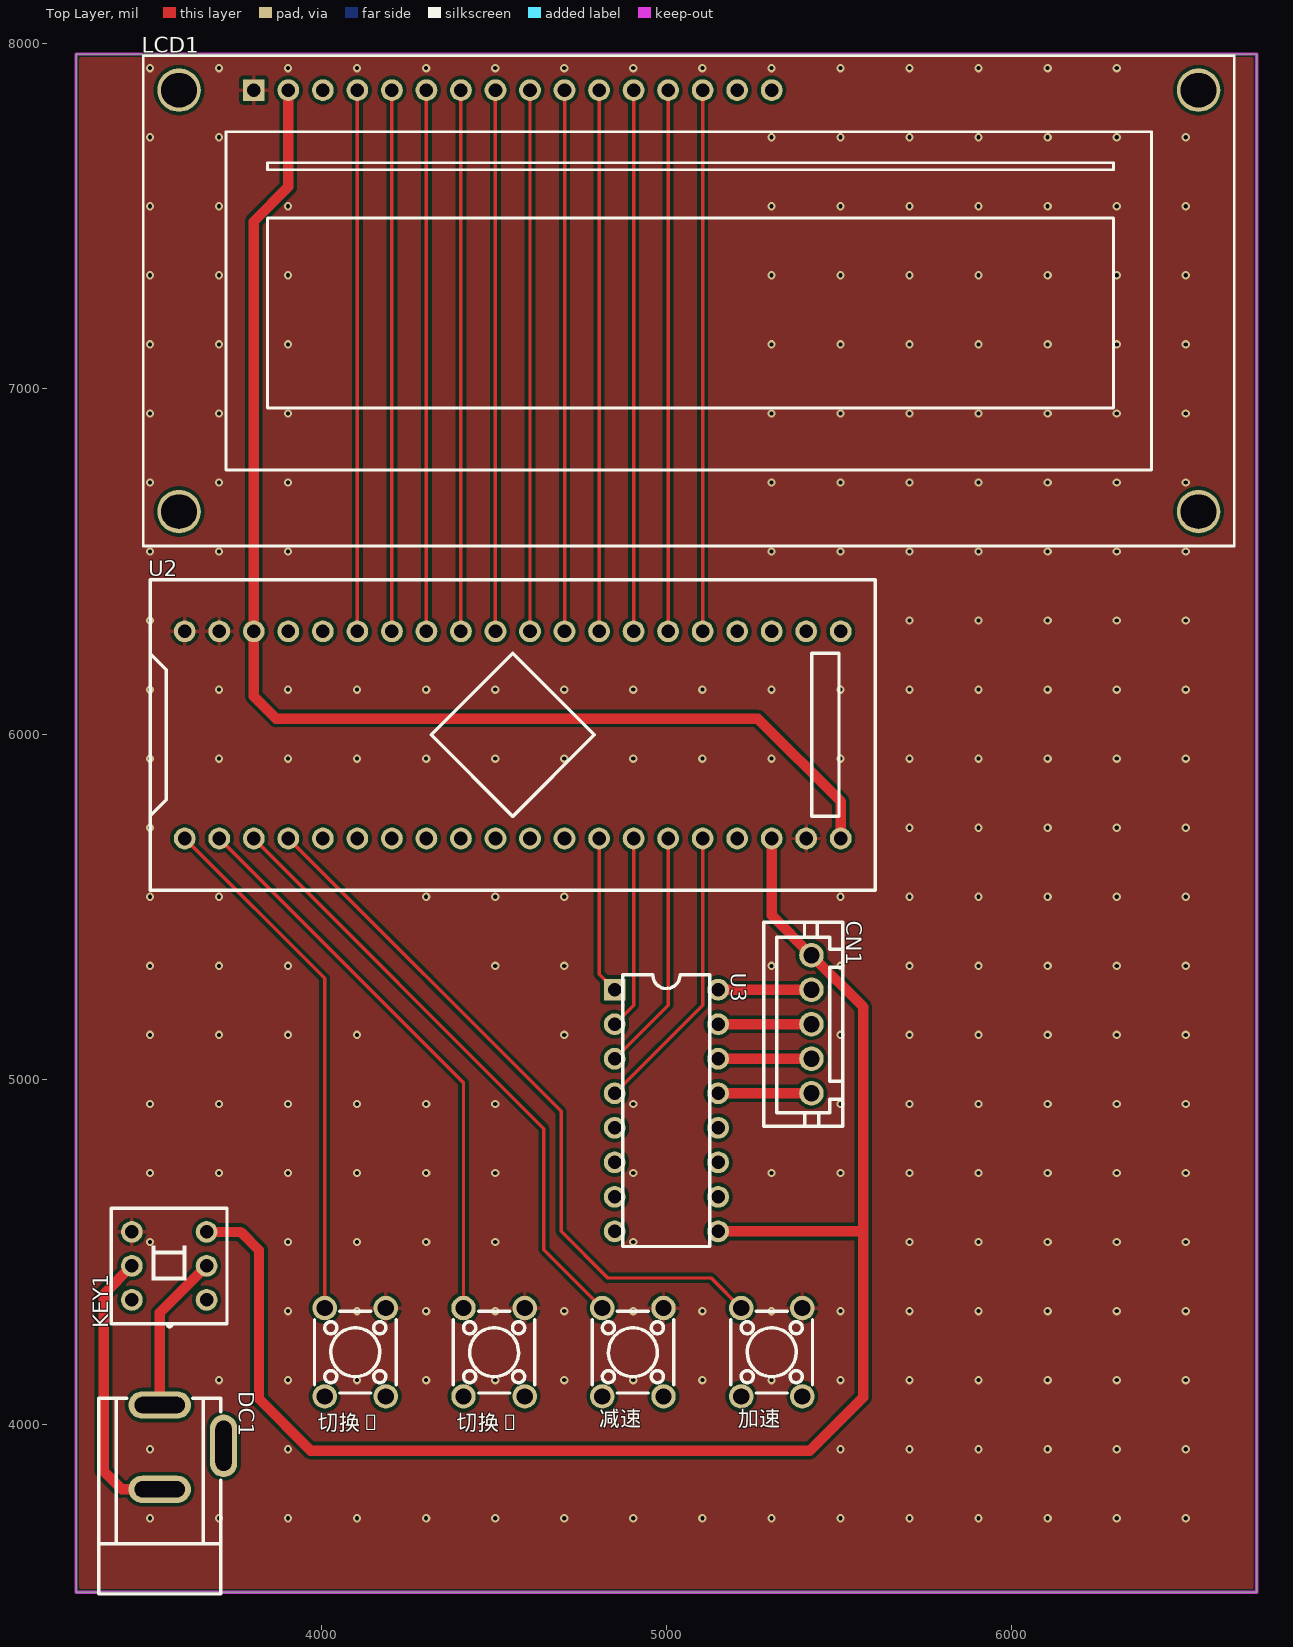
[diagram p0: Top Layer view]
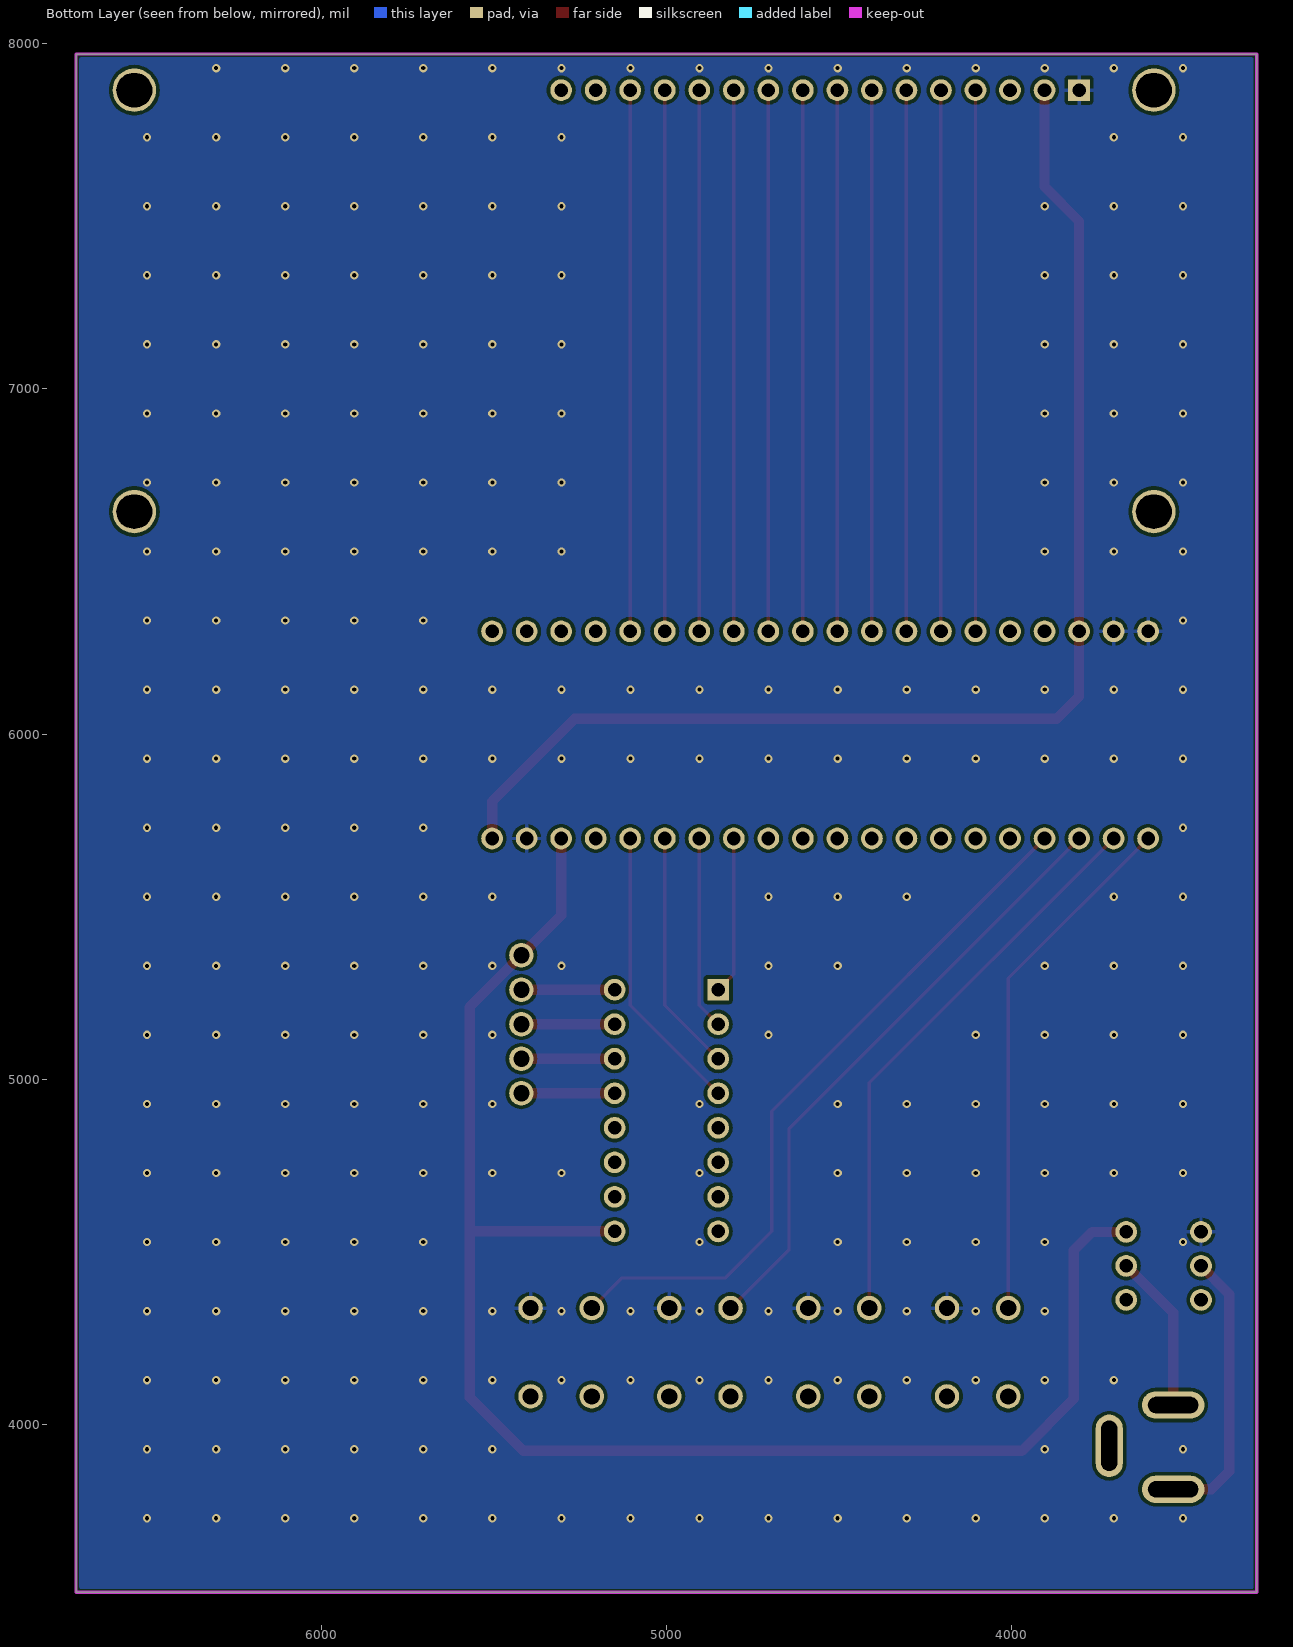
[diagram p1: Bottom Layer view, seen from below]
# Altium PCB MISC51167.pcbdoc
Units mil, origin at the board's own origin, x right, y up, seen from the top; angles counter-clockwise.
Board outline 3420 x 4455 mil, 2 copper layers (Top Layer, Bottom Layer), stack 62.206 mil thick; 10 components, 28 nets, 106 pads, 253 vias.

## Layer stack, top to bottom
Top Solder Mask Layer: solder mask 0.394, Dk 3.3
Top Layer: signal copper 1.379
Dielectric1: surface 59.449, FR4, Dk 4.5
Bottom Layer: signal copper 1.378
Bottom Solder Mask Layer: solder mask 0.394, Dk 3.3

## Board outline
3290,7970 3290,3515 6710,3515 6710,7970

## Design rules (kind name [scope] priority, off if disabled: settings)
BoardOutlineClearance copperThickness2oz_1 [All] p2 off: genericclearance=7.99 ignorepadtopadclearanceinfootprint=FALSE except(0: Arc-SplitContinuation Track-SplitContinuation SMDPad-SplitContinuation THPad-SplitContinuation Via-SplitContinuation Fill-SplitContinuation Region-SplitContinuation Poly-SplitContinuation Text-SplitContinuation Hole-SplitContinuation; 5.98: Arc-CutoutEdge Track-CutoutEdge SMDPad-CutoutEdge THPad-CutoutEdge Via-CutoutEdge Text-CutoutEdge; 6.9: Hole-OutlineEdge Hole-CutoutEdge; 10: Poly-OutlineEdge Poly-CutoutEdge; 11.81: Arc-OutlineEdge Track-OutlineEdge SMDPad-OutlineEdge THPad-OutlineEdge Via-OutlineEdge Fill-OutlineEdge Region-OutlineEdge Text-OutlineEdge Fill-CutoutEdge Region-CutoutEdge)
BoardOutlineClearance Plane_innerPlane_1 [All] p4 off: genericclearance=4.02 ignorepadtopadclearanceinfootprint=FALSE except(0: Arc-SplitContinuation Track-SplitContinuation SMDPad-SplitContinuation THPad-SplitContinuation Via-SplitContinuation Fill-SplitContinuation Region-SplitContinuation Poly-SplitContinuation Text-SplitContinuation Hole-SplitContinuation; 5.98: Arc-CutoutEdge Track-CutoutEdge SMDPad-CutoutEdge THPad-CutoutEdge Via-CutoutEdge Text-CutoutEdge; 6.9: Hole-OutlineEdge Hole-CutoutEdge; 10: Poly-OutlineEdge Poly-CutoutEdge; 11.81: Arc-OutlineEdge Track-OutlineEdge SMDPad-OutlineEdge THPad-OutlineEdge Via-OutlineEdge Fill-OutlineEdge Region-OutlineEdge Text-OutlineEdge Fill-CutoutEdge Region-CutoutEdge)
BoardOutlineClearance Copper_copperRegion_1 [All] p6 off: genericclearance=4.02 ignorepadtopadclearanceinfootprint=FALSE except(0: Arc-SplitContinuation Track-SplitContinuation SMDPad-SplitContinuation THPad-SplitContinuation Via-SplitContinuation Fill-SplitContinuation Region-SplitContinuation Poly-SplitContinuation Text-SplitContinuation Hole-SplitContinuation; 5.98: Arc-CutoutEdge Track-CutoutEdge SMDPad-CutoutEdge THPad-CutoutEdge Via-CutoutEdge Text-CutoutEdge; 6.9: Hole-OutlineEdge Hole-CutoutEdge; 10: Poly-OutlineEdge Poly-CutoutEdge; 11.81: Arc-OutlineEdge Track-OutlineEdge SMDPad-OutlineEdge THPad-OutlineEdge Via-OutlineEdge Fill-OutlineEdge Region-OutlineEdge Text-OutlineEdge Fill-CutoutEdge Region-CutoutEdge)
BoardOutlineClearance copperThickness1oz_1 [All] p8: genericclearance=4.02 ignorepadtopadclearanceinfootprint=FALSE except(0: Arc-SplitContinuation Track-SplitContinuation SMDPad-SplitContinuation THPad-SplitContinuation Via-SplitContinuation Fill-SplitContinuation Region-SplitContinuation Poly-SplitContinuation Text-SplitContinuation Hole-SplitContinuation; 5.98: Arc-CutoutEdge Track-CutoutEdge SMDPad-CutoutEdge THPad-CutoutEdge Via-CutoutEdge Text-CutoutEdge; 6.9: Hole-OutlineEdge Hole-CutoutEdge; 10: Poly-OutlineEdge Poly-CutoutEdge; 11.81: Arc-OutlineEdge Track-OutlineEdge SMDPad-OutlineEdge THPad-OutlineEdge Via-OutlineEdge Fill-OutlineEdge Region-OutlineEdge Text-OutlineEdge Fill-CutoutEdge Region-CutoutEdge)
Clearance copperThickness2oz [All] p1 off: gap=7.99 ignorepadtopadclearanceinfootprint=FALSE except(5.98: SMDPad-Track SMDPad-SMDPad THPad-Track SMDPad-THPad THPad-THPad Track-Via SMDPad-Via THPad-Via Via-Via Fill-SMDPad Region-SMDPad Fill-THPad Region-THPad Fill-Via Region-Via Fill-Fill Fill-Region Region-Region Arc-Track Arc-SMDPad Arc-THPad Arc-Via Fill-Arc Region-Arc Arc-Arc Text-Track SMDPad-Text Text-THPad Text-Via Fill-Text Region-Text Arc-Text Text-Text; 6.9: Hole-Track Hole-SMDPad Hole-THPad Hole-Via Fill-Hole Region-Hole Hole-Arc Hole-Text; 10: Poly-Track Poly-SMDPad Poly-THPad Poly-Via Poly-Fill Poly-Region Poly-Poly Poly-Arc Poly-Text Poly-Hole; 11.81: Fill-Track Region-Track)
Clearance Plane_innerPlane [All] p3 off: gap=4.02 ignorepadtopadclearanceinfootprint=FALSE except(5.98: SMDPad-Track SMDPad-SMDPad THPad-Track SMDPad-THPad THPad-THPad Track-Via SMDPad-Via THPad-Via Via-Via Fill-SMDPad Region-SMDPad Fill-THPad Region-THPad Fill-Via Region-Via Fill-Fill Fill-Region Region-Region Arc-Track Arc-SMDPad Arc-THPad Arc-Via Fill-Arc Region-Arc Arc-Arc Text-Track SMDPad-Text Text-THPad Text-Via Fill-Text Region-Text Arc-Text Text-Text; 6.9: Hole-Track Hole-SMDPad Hole-THPad Hole-Via Fill-Hole Region-Hole Hole-Arc Hole-Text; 10: Poly-Track Poly-SMDPad Poly-THPad Poly-Via Poly-Fill Poly-Region Poly-Poly Poly-Arc Poly-Text Poly-Hole; 11.81: Fill-Track Region-Track)
Clearance Copper_copperRegion [All] p5 off: gap=4.02 ignorepadtopadclearanceinfootprint=FALSE except(5.98: SMDPad-Track SMDPad-SMDPad THPad-Track SMDPad-THPad THPad-THPad Track-Via SMDPad-Via THPad-Via Via-Via Fill-SMDPad Region-SMDPad Fill-THPad Region-THPad Fill-Via Region-Via Fill-Fill Fill-Region Region-Region Arc-Track Arc-SMDPad Arc-THPad Arc-Via Fill-Arc Region-Arc Arc-Arc Text-Track SMDPad-Text Text-THPad Text-Via Fill-Text Region-Text Arc-Text Text-Text; 6.9: Hole-Track Hole-SMDPad Hole-THPad Hole-Via Fill-Hole Region-Hole Hole-Arc Hole-Text; 10: Poly-Track Poly-SMDPad Poly-THPad Poly-Via Poly-Fill Poly-Region Poly-Poly Poly-Arc Poly-Text Poly-Hole; 11.81: Fill-Track Region-Track)
Clearance copperThickness1oz [All] p7: gap=4.02 ignorepadtopadclearanceinfootprint=FALSE except(5.98: SMDPad-Track SMDPad-SMDPad THPad-Track SMDPad-THPad THPad-THPad Track-Via SMDPad-Via THPad-Via Via-Via Fill-SMDPad Region-SMDPad Fill-THPad Region-THPad Fill-Via Region-Via Fill-Fill Fill-Region Region-Region Arc-Track Arc-SMDPad Arc-THPad Arc-Via Fill-Arc Region-Arc Arc-Arc Text-Track SMDPad-Text Text-THPad Text-Via Fill-Text Region-Text Arc-Text Text-Text; 6.9: Hole-Track Hole-SMDPad Hole-THPad Hole-Via Fill-Hole Region-Hole Hole-Arc Hole-Text; 10: Poly-Track Poly-SMDPad Poly-THPad Poly-Via Poly-Fill Poly-Region Poly-Poly Poly-Arc Poly-Text Poly-Hole; 11.81: Fill-Track Region-Track)
DiffPairsRouting differentialPair [All] p1: maxlimit=6 minlimit=6 mostfreqgap=6 toplayer_minwidth=5 toplayer_prefwidth=10 toplayer_maxwidth=100 toplayer_mingap=6 toplayer_prefgap=6 toplayer_maxgap=6 bottomlayer_minwidth=5 bottomlayer_prefwidth=10 bottomlayer_maxwidth=100 bottomlayer_mingap=6 bottomlayer_prefgap=6 bottomlayer_maxgap=6 maxuncoupledlength=10
HoleToHoleClearance otherClearance [All] p1: gap=11.81 allowstackedmicrovias=TRUE
Length netLength [All] p1: minlimit=0 maxlimit=0
PasteMaskExpansion pasteMaskExpansion [All] p1: expansion=0
PlaneConnect innerPlane [All] p1: planeconnectstyle=Relief reliefexpansion=20 reliefentries=4 reliefconductorwidth=10 reliefairgap=10
PolygonConnect copperRegion [All] p1: connectstyle=Relief reliefconductorwidth=10 reliefentries=4 polygonreliefangle="90 Angle" airgapwidth=10 via.connectstyle=Relief via.reliefconductorwidth=10 via.reliefentries=4 via.polygonreliefangle="90 Angle" via.airgapwidth=10
RoutingVias viaSize [All] p1: holewidth=12.01 width=24.02 viastyle="Through Hole" minholewidth=11.81 minwidth=19.68 maxholewidth=248.03 maxwidth=393.7
SolderMaskExpansion solderMaskExpansion [IsVia] p1: expansion=-1000 istentingtop=TRUE
SolderMaskExpansion solderMaskExpansion [All] p2: expansion=2 istentingtop=FALSE
Width copperThickness2oz_2 [All] p1 off: maxlimit=100 minlimit=8 preferedwidth=10
Width copperThickness1oz_2 [All] p2: maxlimit=100 minlimit=5 preferedwidth=10

## Components (designator, comment, footprint, x,y, rotation, side; value= is the part's Value field where it differs from the comment)
CN1 "XH2.54-5P" CONN-TH_5P-P2.54_C9900008095 5420,5160 r270 top
DC1 "" DC-005_2.5 3545,3930 r270 top
KEY1 "Non-latching switch 8.5×8.5, silent" SW-TH_6P-L8.5-W8.5-P2.54 3560,4460 r90 top
LCD1 "LMB162ADC" LCD1602 5064.72,7255 r0 top
U2 "STM32F103C8T6-Card" CONN-TH_L53.3-W22.9_STM32F103C8T6-CARD 4554.87,5997.94 r0 top
U3 "ULN2003AN" DIP-16_L19.8-W6.5-P2.54-LS7.6-BL 5000,4910 r270 top
减速 "" SW-TH_4P-L6.0-W6.0-P4.50-LS6.5 4902.94,4210 r270 top
切换1 "" SW-TH_4P-L6.0-W6.0-P4.50-LS6.5 4098.81,4210 r270 top
切换2 "" SW-TH_4P-L6.0-W6.0-P4.50-LS6.5 4500.87,4210 r270 top
加速 "" SW-TH_4P-L6.0-W6.0-P4.50-LS6.5 5305,4210 r270 top

## Footprints (in the part's own frame and the unit in brackets; to place one, negate y for a bottom-side part, rotate by r counter-clockwise, add the part's x,y. Pads: shape width x height; smd on the part's side, far side on the other; paste and mask are expansions set on the pad)
CONN-TH_5P-P2.54_C9900008095 [mm]
  round 1.8 hole 1.2 paste+0 mask+0.05: 1(-5.08,0) 2(-2.54,0) 3(0,0) 5(5.08,0)
  round 1.8 hole 1.2 copper offset 0,0 paste+0 mask+0.05: 4(2.54,0)
  silkscreen extent -7.5,-3.5 7.5,2.3
CONN-TH_L53.3-W22.9_STM32F103C8T6-CARD [mm]
  round 1.6 hole 1: 1(-24.13,-7.62) 2(-21.59,-7.62) 3(-19.05,-7.62) 4(-16.51,-7.62) 5(-13.97,-7.62) 6(-11.43,-7.62) 7(-8.89,-7.62) 8(-6.35,-7.62) 9(-3.81,-7.62) 10(-1.27,-7.62) 11(1.27,-7.62) 12(3.81,-7.62) 13(6.35,-7.62) 14(8.89,-7.62) 15(11.43,-7.62) 16(13.97,-7.62) 17(16.51,-7.62) 18(19.05,-7.62) 19(21.59,-7.62) 20(24.13,-7.62) 21(24.13,7.62) 22(21.59,7.62) 23(19.05,7.62) 24(16.51,7.62) 25(13.97,7.62) 26(11.43,7.62) 27(8.89,7.62) 28(6.35,7.62) 29(3.81,7.62) 30(1.27,7.62) 31(-1.27,7.62) 32(-3.81,7.62) 33(-6.35,7.62) 34(-8.89,7.62) 35(-11.43,7.62) 36(-13.97,7.62) 37(-16.51,7.62) 38(-19.05,7.62) 39(-21.59,7.62) 40(-24.13,7.62)
  silkscreen extent -26.67,-11.43 26.67,11.43
DC-005_2.5 [mm]
  oval 2x4.6 hole 1.2 slot 3.7 at 90 deg paste+0 mask+0.051: 1(-3.227,-0.318) 2(2.973,-0.318)
  oval 4.6x2 hole 1.2 slot 3.7 at 0 deg paste+0 mask+0.051: 3(-0.227,4.382)
  silkscreen extent -3.73,-4.82 10.67,4.18
DIP-16_L19.8-W6.5-P2.54-LS7.6-BL [mm]
  rect 1.6x1.6 hole 1: 1(-8.89,-3.81)
  round 1.6 hole 1 copper offset 0,0: 2(-6.35,-3.81) 3(-3.81,-3.81) 4(-1.27,-3.81) 5(1.27,-3.81) 6(3.81,-3.81) 7(6.35,-3.81) 8(8.89,-3.81) 9(8.89,3.81) 10(6.35,3.81) 11(3.81,3.81) 12(1.27,3.81) 13(-1.27,3.81) 14(-3.81,3.81) 15(-6.35,3.81) 16(-8.89,3.81)
  silkscreen extent -10,-3.2 10,3.2
LCD1602 [mm]
  round 3.2 hole 2.5 slot 2.625 at 0 deg: 0(-37.5,-15.5) 0(-37.5,15.5) 0(37.5,-15.5) 0(37.5,15.5)
  rect 1.6x1.6 hole 1: 1(-32,15.5)
  round 1.6 hole 1: 2(-29.46,15.5) 3(-26.92,15.5) 4(-24.38,15.5) 5(-21.84,15.5) 6(-19.3,15.5) 7(-16.76,15.5) 8(-14.22,15.5) 9(-11.68,15.5) 10(-9.14,15.5) 11(-6.6,15.5) 12(-4.06,15.5) 13(-1.52,15.5) 14(1.02,15.5) 15(3.56,15.5) 16(6.1,15.5)
  silkscreen extent -40.13,-18.03 40.13,18.03
SW-TH_4P-L6.0-W6.0-P4.50-LS6.5 [mm]
  round 1.8 hole 1.2: 1(-3.25,2.25) 2(3.25,2.25) 3(-3.25,-2.25) 4(3.25,-2.25)
  silkscreen extent -3,-3 3,3
SW-TH_6P-L8.5-W8.5-P2.54 [mm]
  round 1.6 hole 1: 1(-2.5,-2.75) 2(0,-2.75) 3(2.5,-2.75) 4(-2.5,2.75) 5(0,2.75) 6(2.5,2.75)
  silkscreen extent -4.47,-4.25 4.25,4.25

## Via types
v1: diameter 24.02, hole 12, Top Layer to Bottom Layer, 253 vias

## Nets (pads, with @x,y where several pads share a name; then routed paths per layer and width w, separated by ;. In a path a pad name is that pad's centre, name@x,y a point inside that pad or via, vN(x,y) a via of type N, cw(c..) or ccw(c..) an arc to the next point about the centre after c; other vN are vias at no path point)
$1N579: LCD1.14 U2.25 | length 1567.3
  Top Layer w10: U2.25 LCD1.14
$1N584: LCD1.13 U2.26 | length 1567.3
  Top Layer w10: U2.26 LCD1.13
$1N590: LCD1.12 U2.27 | length 1567.3
  Top Layer w10: U2.27 LCD1.12
$1N596: LCD1.11 U2.28 | length 1567.3
  Top Layer w10: U2.28 LCD1.11
$1N608: LCD1.10 U2.29 | length 1567.3
  Top Layer w10: U2.29 LCD1.10
$1N613: LCD1.9 U2.30 | length 1567.3
  Top Layer w10: U2.30 LCD1.9
$1N619: LCD1.8 U2.31 | length 1567.3
  Top Layer w10: U2.31 LCD1.8
$1N625: LCD1.7 U2.32 | length 1567.3
  Top Layer w10: U2.32 LCD1.7
$1N1244: CN1.5 U3.13 | length 270
  Top Layer w30: U3.13 CN1.5
$1N1246: CN1.4 U3.14 | length 270
  Top Layer w30: U3.14 CN1.4
$1N1248: CN1.3 U3.15 | length 270
  Top Layer w30: U3.15 CN1.3
$1N1250: CN1.2 U3.16 | length 270
  Top Layer w30: U3.16 CN1.2
$1N1801: DC1.2 KEY1.5 | length 812.9
  Top Layer w30: KEY1.5 3370,4378.27 3370,3865 3422.04,3812.96 DC1.2
$1N1803: DC1.1 KEY1.2 | length 459.2
  Top Layer w30: DC1.1 3532.49,4324.21 KEY1.2
+5V: CN1.1 KEY1.3 U2.18 U3.9 | length 4628
  Top Layer w30: KEY1.3 3766.57,4558.43 3820,4505 3820,4075 3970,3925 5415,3925 5570,4080 5570,4560 ; U3.9 5570,4560 ; U2.18 5304.88,5475.12 CN1.1 5570,5210 5570,4560
A: U2.13 U3.1 | length 456.6
  Top Layer w10: U2.13 4804.88,5305.12 U3.1
B: U2.14 U3.2 | length 560.7
  Top Layer w10: U3.2 4904.88,5214.88 U2.14
C: U2.15 U3.3 | length 702.1
  Top Layer w10: U3.3 5004.88,5214.88 U2.15
D: U2.16 U3.4 | length 843.5
  Top Layer w10: U3.4 5104.88,5214.88 U2.16
EN: LCD1.6 U2.33 | length 1567.3
  Top Layer w10: U2.33 LCD1.6
GND: KEY1.6 LCD1.1 U2.19 U2.39 U2.40 减速.1 切换1.1 切换2.1 加速.1
  other v1: 3504.1,3729.1 3704.1,3729.1 3904.1,3729.1 4104.1,3729.1 4304.1,3729.1 4504.1,3729.1 4704.1,3729.1 4904.1,3729.1 5104.1,3729.1 5304.1,3729.1 5504.1,3729.1 5704.1,3729.1 5904.1,3729.1 6104.1,3729.1 6304.1,3729.1 6504.1,3729.1 3504.1,3929.1 3904.1,3929.1 5504.1,3929.1 5704.1,3929.1 5904.1,3929.1 6104.1,3929.1 6304.1,3929.1 6504.1,3929.1 3704.1,4129.1 3904.1,4129.1 4104.1,4129.1 4304.1,4129.1 4504.1,4129.1 4704.1,4129.1 4904.1,4129.1 5104.1,4129.1 5304.1,4129.1 5504.1,4129.1 5704.1,4129.1 5904.1,4129.1 6104.1,4129.1 6304.1,4129.1 6504.1,4129.1 3904.1,4329.1 4104.1,4329.1 4304.1,4329.1 4504.1,4329.1 4704.1,4329.1 4904.1,4329.1 5104.1,4329.1 5304.1,4329.1 5504.1,4329.1 5704.1,4329.1 5904.1,4329.1 6104.1,4329.1 6304.1,4329.1 6504.1,4329.1 3504.1,4529.1 3904.1,4529.1 4104.1,4529.1 4304.1,4529.1 4504.1,4529.1 4904.1,4529.1 5704.1,4529.1 5904.1,4529.1 6104.1,4529.1 6304.1,4529.1 6504.1,4529.1 3504.1,4729.1 3704.1,4729.1 3904.1,4729.1 4104.1,4729.1 4304.1,4729.1 4504.1,4729.1 4904.1,4729.1 5304.1,4729.1 5504.1,4729.1 5704.1,4729.1 5904.1,4729.1 6104.1,4729.1 6304.1,4729.1 6504.1,4729.1 3504.1,4929.1 3704.1,4929.1 3904.1,4929.1 4104.1,4929.1 4304.1,4929.1 4504.1,4929.1 4904.1,4929.1 5504.1,4929.1 5704.1,4929.1 5904.1,4929.1 6104.1,4929.1 6304.1,4929.1 6504.1,4929.1 3504.1,5129.1 3704.1,5129.1 3904.1,5129.1 4104.1,5129.1 4704.1,5129.1 5504.1,5129.1 5704.1,5129.1 5904.1,5129.1 6104.1,5129.1 6304.1,5129.1 6504.1,5129.1 3504.1,5329.1 3704.1,5329.1 3904.1,5329.1 4504.1,5329.1 4704.1,5329.1 5304.1,5329.1 5504.1,5329.1 5704.1,5329.1 5904.1,5329.1 6104.1,5329.1 6304.1,5329.1 6504.1,5329.1 3504.1,5529.1 3704.1,5529.1 4304.1,5529.1 4504.1,5529.1 4704.1,5529.1 5504.1,5529.1 5704.1,5529.1 5904.1,5529.1 6104.1,5529.1 6304.1,5529.1 6504.1,5529.1 3504.1,5729.1 5704.1,5729.1 5904.1,5729.1 6104.1,5729.1 6304.1,5729.1 6504.1,5729.1 3504.1,5929.1 3704.1,5929.1 3904.1,5929.1 4104.1,5929.1 4304.1,5929.1 4504.1,5929.1 4704.1,5929.1 4904.1,5929.1 5104.1,5929.1 5304.1,5929.1 5504.1,5929.1 5704.1,5929.1 5904.1,5929.1 6104.1,5929.1 6304.1,5929.1 6504.1,5929.1 3504.1,6129.1 3704.1,6129.1 3904.1,6129.1 4104.1,6129.1 4304.1,6129.1 4504.1,6129.1 4704.1,6129.1 4904.1,6129.1 5104.1,6129.1 5304.1,6129.1 5504.1,6129.1 5704.1,6129.1 5904.1,6129.1 6104.1,6129.1 6304.1,6129.1 6504.1,6129.1 3504.1,6329.1 5704.1,6329.1 5904.1,6329.1 6104.1,6329.1 6304.1,6329.1 6504.1,6329.1 3504.1,6529.1 3704.1,6529.1 3904.1,6529.1 5304.1,6529.1 5504.1,6529.1 5704.1,6529.1 5904.1,6529.1 6104.1,6529.1 6304.1,6529.1 6504.1,6529.1 3504.1,6729.1 3704.1,6729.1 3904.1,6729.1 5304.1,6729.1 5504.1,6729.1 5704.1,6729.1 5904.1,6729.1 6104.1,6729.1 6304.1,6729.1 6504.1,6729.1 3504.1,6929.1 3704.1,6929.1 3904.1,6929.1 5304.1,6929.1 5504.1,6929.1 5704.1,6929.1 5904.1,6929.1 6104.1,6929.1 6304.1,6929.1 6504.1,6929.1 3504.1,7129.1 3704.1,7129.1 3904.1,7129.1 5304.1,7129.1 5504.1,7129.1 5704.1,7129.1 5904.1,7129.1 6104.1,7129.1 6304.1,7129.1 6504.1,7129.1 3504.1,7329.1 3704.1,7329.1 3904.1,7329.1 5304.1,7329.1 5504.1,7329.1 5704.1,7329.1 5904.1,7329.1 6104.1,7329.1 6304.1,7329.1 6504.1,7329.1 3504.1,7529.1 3704.1,7529.1 3904.1,7529.1 5304.1,7529.1 5504.1,7529.1 5704.1,7529.1 5904.1,7529.1 6104.1,7529.1 6304.1,7529.1 6504.1,7529.1 3504.1,7729.1 3704.1,7729.1 5304.1,7729.1 5504.1,7729.1 5704.1,7729.1 5904.1,7729.1 6104.1,7729.1 6304.1,7729.1 6504.1,7729.1 3504.1,7929.1 3704.1,7929.1 3904.1,7929.1 4104.1,7929.1 4304.1,7929.1 4504.1,7929.1 4704.1,7929.1 4904.1,7929.1 5104.1,7929.1 5304.1,7929.1 5504.1,7929.1 5704.1,7929.1 5904.1,7929.1 6104.1,7929.1 6304.1,7929.1
K1: U2.1 切换1.3 | length 1527.9
  Top Layer w10: U2.1 4010.23,5292.59 切换1.3
K2: U2.2 切换2.3 | length 1653
  Top Layer w10: U2.2 4412.29,4990.53 切换2.3
K3: U2.3 减速.3 | length 1778.1
  Top Layer w10: U2.3 4645,4857.82 4645,4507.31 减速.3
K4: U2.4 加速.3 | length 2078.6
  Top Layer w10: U2.4 4695,4907.82 4695,4560 4830,4425 5129.37,4425 加速.3
RS: LCD1.4 U2.35 | length 1567.3
  Top Layer w10: U2.35 LCD1.4
RW: LCD1.5 U2.34 | length 1567.3
  Top Layer w10: U2.34 LCD1.5
VCC: LCD1.2 U2.20 U2.38 | length 3730.1
  Top Layer w30: LCD1.2 3904.88,7584.88 3804.88,7484.88 U2.38 3804.88,6110.12 3870,6045 5265,6045 5504.88,5805.12 U2.20
pads on no net: DC1.3 KEY1.1 KEY1.4 LCD1.0 LCD1.3 LCD1.15 LCD1.16 U2.5 U2.6 U2.7 U2.8 U2.9 U2.10 U2.11 U2.12 U2.17 U2.21 U2.22 U2.23 U2.24 U2.36 U2.37 U3.5 U3.6 U3.7 U3.8 U3.10 U3.11 U3.12 减速.2 减速.4 切换1.2 切换1.4 切换2.2 切换2.4 加速.2 加速.4

## Polygon pours and split planes (outlines as drawn)
GND on Top Layer (solid, remove dead copper, pour order 0): 3000,8270 3000,3000 7350,3000 7350,8270
GND on Bottom Layer (solid, remove dead copper, pour order 2): 3170,8320 3170,3260 7240,3260 7240,8320

## Keep-outs
Board Outline Layer:
  the board outline again, w10